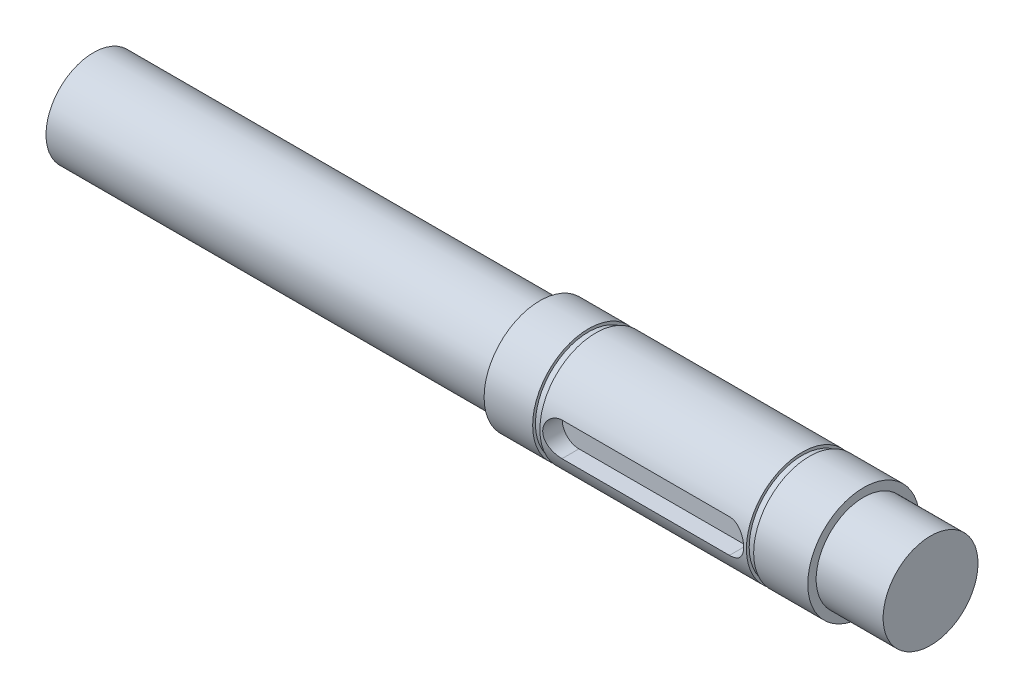
from build123d import *

# Parameters (mm, degrees)
SKETCH_1_R          = 10
EXTRUDE_1_DEPTH     = 58
SKETCH_2_R          = 8.5
EXTRUDE_2_DEPTH     = 12
EXTRUDE_START       = 80
SKETCH_3_R          = 8.5
EXTRUDE_3_DEPTH     = 80
CUT_EXTRUDE_1_DEPTH = 83.29368141
SKETCH_5_W          = 1.3
SKETCH_5_H          = 0.5


with BuildPart() as part:
    # 草图1 → 凸台-拉伸1 (new body)
    with BuildSketch(Plane(origin=(0, 0, 0), x_dir=(0, 0, -1), z_dir=(1, 0, 0))):
        with Locations(Location((0, 0, 0), (0, 0, 180))):
            Circle(SKETCH_1_R)
    extrude(amount=EXTRUDE_1_DEPTH)

    # 草图2 → 凸台-拉伸2 (add)
    with BuildSketch(Plane(origin=(58, 0, 0), x_dir=(0, 0, -1), z_dir=(1, 0, 0))):
        Circle(SKETCH_2_R)
    extrude(amount=EXTRUDE_2_DEPTH)

    # 草图3 → 凸台-拉伸3 (add)
    with BuildSketch(Plane.ZY.offset(EXTRUDE_START)):
        with Locations(Location((0, 0, 0), (0, 0, 180))):
            Circle(SKETCH_3_R)
    extrude(amount=-EXTRUDE_3_DEPTH)

    # 草图4 → 切除-拉伸1 (cut, through all)
    with BuildSketch(Plane.XY.offset(6.5)):
        with BuildLine():
            Line((13.5, 3), (43.5, 3))
            ThreePointArc((43.5, 3), (46.5, 0), (43.5, -3))
            Line((43.5, -3), (13.5, -3))
            ThreePointArc((13.5, -3), (10.5, 0), (13.5, 3))
        make_face()
    extrude(amount=CUT_EXTRUDE_1_DEPTH, mode=Mode.SUBTRACT)

    # 草图5 → 切除-旋转1 (revolve, cut)
    with BuildSketch(Plane(origin=(0, 0, 0), x_dir=(1, 0, 0), z_dir=(0, 1, 0)), mode=Mode.PRIVATE) as cut_revolve_1_sk:
        with Locations((9.35, 9.75)):
            Rectangle(SKETCH_5_W, SKETCH_5_H)
        with Locations((47.65, 9.75)):
            Rectangle(SKETCH_5_W, SKETCH_5_H)
    revolve(cut_revolve_1_sk.sketch.rotate(Axis((0, 0, 0), (1, 0, 0)), 180), axis=Axis((0, 0, 0), (1, 0, 0)), mode=Mode.SUBTRACT)


solid = part.part
